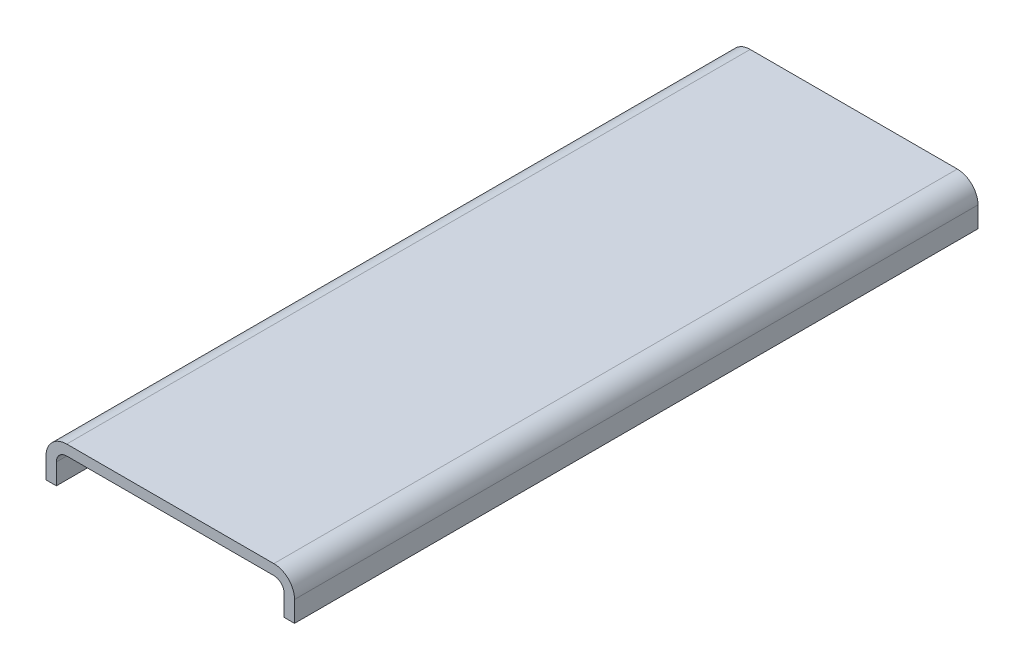
from build123d import *

# Parameters (mm, degrees)
EXTRUDE_1_DEPTH = 320
EXTRUDE_START   = 10
EXTRUDE_2_DEPTH = 10


with BuildPart() as part:
    # 草图1 → 凸台-拉伸1 (new body)
    with BuildSketch(Plane.XY):
        with BuildLine():
            Line((10, 0), (110, 0))
            ThreePointArc((110, 0), (117.071067812, -2.928932188), (120, -10))
            Line((120, -10), (120, -20))
            Line((120, -20), (115, -20))
            Line((115, -20), (115, -10))
            ThreePointArc((115, -10), (113.535533906, -6.464466094), (110, -5))
            Line((110, -5), (10, -5))
            ThreePointArc((10, -5), (6.464466094, -6.464466094), (5, -10))
            Line((5, -10), (5, -20))
            Line((5, -20), (0, -20))
            Line((0, -20), (0, -10))
            ThreePointArc((0, -10), (2.928932188, -2.928932188), (10, 0))
        make_face()
    extrude(amount=EXTRUDE_1_DEPTH)

    # 草图2 → 凸台-拉伸2 (add)
    with BuildSketch(Plane(origin=(0, 0, 0), x_dir=(-1, 0, 0), z_dir=(0, 0, -1)).offset(EXTRUDE_START)):
        with BuildLine():
            Line((-120, -20), (-115, -20))
            Line((-115, -20), (-115, -10))
            ThreePointArc((-115, -10), (-113.535533906, -6.464466094), (-110, -5))
            Line((-110, -5), (-10, -5))
            ThreePointArc((-10, -5), (-6.464466094, -6.464466094), (-5, -10))
            Line((-5, -10), (-5, -20))
            Line((-5, -20), (0, -20))
            Line((0, -20), (0, -10))
            ThreePointArc((0, -10), (-2.928932188, -2.928932188), (-10, 0))
            Line((-10, 0), (-110, 0))
            ThreePointArc((-110, 0), (-117.071067812, -2.928932188), (-120, -10))
            Line((-120, -10), (-120, -20))
        make_face()
    extrude(amount=-EXTRUDE_2_DEPTH)


solid = part.part
